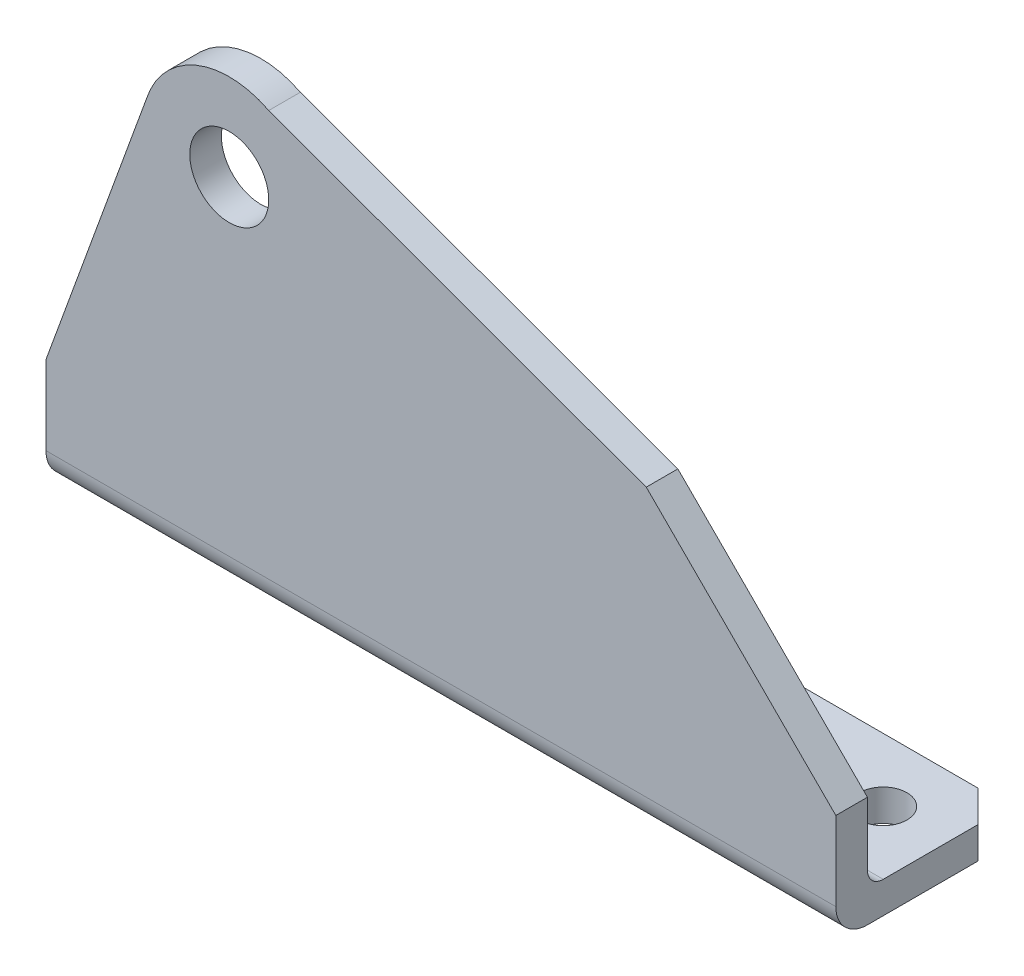
SolidWorks part; units mm, degrees
material "1023 碳钢板 (SS)"
ref_plane "Front Plane" through (0, 0, 0) normal (0, 0, 1) x (1, 0, 0)
ref_plane "Top Plane" through (0, 0, 0) normal (0, 1, 0) x (1, 0, 0)
ref_plane "Right Plane" through (0, 0, 0) normal (1, 0, 0) x (0, 0, -1)
sketch "Sketch1" plane through (0, 0, 0) normal (0, 0, 1) x (1, 0, 0)
  line L1 (125, 90.5) -> (-125, 90.5)
  line L2 (125, 90.5) -> (125, -90.5)
  line L3 (125, -90.5) -> (-125, -90.5)
  line L4 (-125, 90.5) -> (-125, -90.5)
  line L5 (125, 90.5) -> (-125, -90.5) construction
  line L6 (125, -90.5) -> (-125, 90.5) construction
  point P0 (0, 0)
  dimension "D1" = 250
  dimension "D2" = 181
extrude "Boss-Extrude1" add sketch "Sketch1" along normal blind 10 contours L2 L1 L4 L3
sketch "Sketch2" plane through (0, 0, 10) normal (0, 0, 1) x (1, 0, 0)
  line L0 (-125, -55.5) -> (-93.1599, 31.98)
  line L1 (-125, 90.5) -> (-125, -90.5) construction
  line L2 (125, -90.5) -> (-125, -90.5) construction
  line L3 (125, -55.5) -> (65, 4.5)
  line L4 (125, 90.5) -> (125, -90.5) construction
  line L5 (65, 4.5) -> (-54.4969, 47.9933)
  line L6 (-125, -55.5) -> (-125, -90.5)
  line L7 (-125, -90.5) -> (125, -90.5)
  line L8 (125, -90.5) -> (125, -55.5)
  arc A0 (-54.4969, 47.9933) -> (-93.1599, 31.98) centre (-67, 23.5) ccw
  dimension "D4" = 55
  dimension "D5" = 58
  dimension "D1" = 35
  dimension "D2" = 70
  dimension "D3" = 114
  dimension "D6" = 35
  dimension "D7" = 60
  dimension "D8" = 60
  dimension "D9" = 90
extrude "Cut-Extrude1" cut sketch "Sketch2" against normal blind 10 flip side to cut
sketch "Sketch3" plane through (0, 0, 10) normal (0, 0, 1) x (1, 0, 0)
  line L0 (125, -90.5) -> (-125, -90.5) construction
  line L1 (-125, -55.5) -> (-125, -90.5) construction
  circle A0 centre (-67, 23.5) radius 12.5
  dimension "D1" = 25
  dimension "D3" = 58
  dimension "D2" = 114
extrude "Cut-Extrude2" cut sketch "Sketch3" against normal blind 10
sketch "Sketch4" plane through (0, 0, 0) normal (0, 0, -1) x (-1, 0, 0)
  line L0 (-125, -80.5) -> (125, -80.5)
  line L1 (-125, -55.5) -> (-125, -90.5) construction
  line L2 (125, -55.5) -> (125, -90.5) construction
  line L3 (125, -80.5) -> (125, -90.5)
  line L4 (125, -90.5) -> (-125, -90.5)
  line L5 (-125, -90.5) -> (-125, -80.5)
  dimension "D1" = 10
extrude "Boss-Extrude2" add sketch "Sketch4" along normal blind 45
fillet "Fillet1" radius 10 1 edges at (0, -90.5, 10)
fillet "Fillet2" radius 5 1 edges at (0, -80.5, 0)
sketch "Sketch5" plane through (0, -90.5, 0) normal (0, -1, 0) x (1, 0, 0)
  line L0 (-125, 0) -> (-125, -45) construction
  line L2 (-125, 10) -> (125, 10) construction
  circle A0 centre (-105, -25) radius 7.5
  circle A1 centre (105, -25) radius 7.5
  dimension "D1" = 210
  dimension "D3" = 15
  dimension "D4" = 35
  dimension "D2" = 20
extrude "Cut-Extrude3" cut sketch "Sketch5" against normal blind 45
chamfer "Chamfer1" distance 10 angle 45 2 edges at (125, -85.5, -45) (-125, -85.5, -45)
